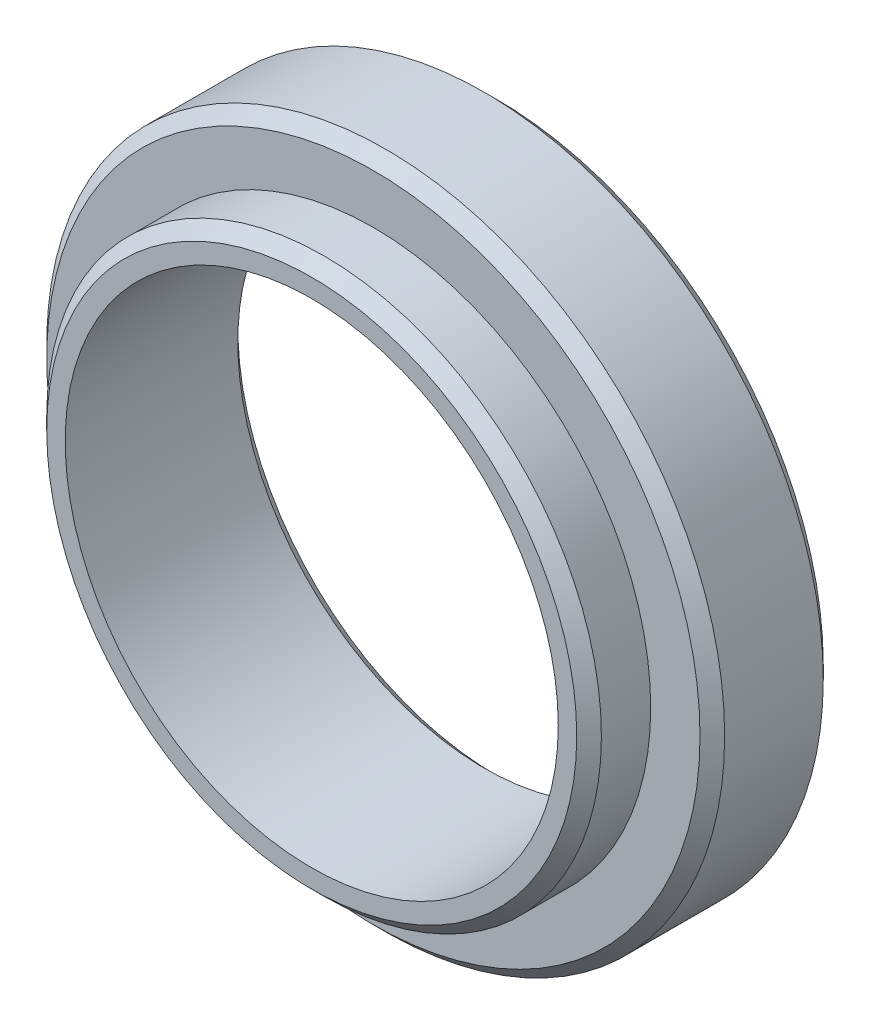
from build123d import *

# Parameters (mm, degrees)
SKETCH1_R           = 27.5
SKETCH1_R_2         = 20
BOSS_EXTRUDE1_DEPTH = 15
CUT_EXTRUDE1_START  = -5
SKETCH2_R           = 27.5
SKETCH2_R_2         = 22.5
CUT_EXTRUDE1_DEPTH  = 5
CHAMFER1_SIZE       = 1


with BuildPart() as part:
    # Sketch1 → Boss-Extrude1 (new body)
    with BuildSketch(Plane.XY):
        Circle(SKETCH1_R)
        Circle(SKETCH1_R_2, mode=Mode.SUBTRACT)
    extrude(amount=BOSS_EXTRUDE1_DEPTH)

    # Sketch2 → Cut-Extrude1 (cut)
    with BuildSketch(Plane.XY.offset(15).offset(CUT_EXTRUDE1_START)):
        Circle(SKETCH2_R)
        Circle(SKETCH2_R_2, mode=Mode.SUBTRACT)
    extrude(amount=CUT_EXTRUDE1_DEPTH, mode=Mode.SUBTRACT)

    # Chamfer1
    chamfer1_edges = [part.edges().sort_by_distance(p)[0] for p in [
        (-27.5, 0, 10),
        (-22.5, 0, 15),
        (-27.5, 0, 0),
        (-20, 0, 0),
    ]]
    chamfer(chamfer1_edges, length=CHAMFER1_SIZE)


solid = part.part
